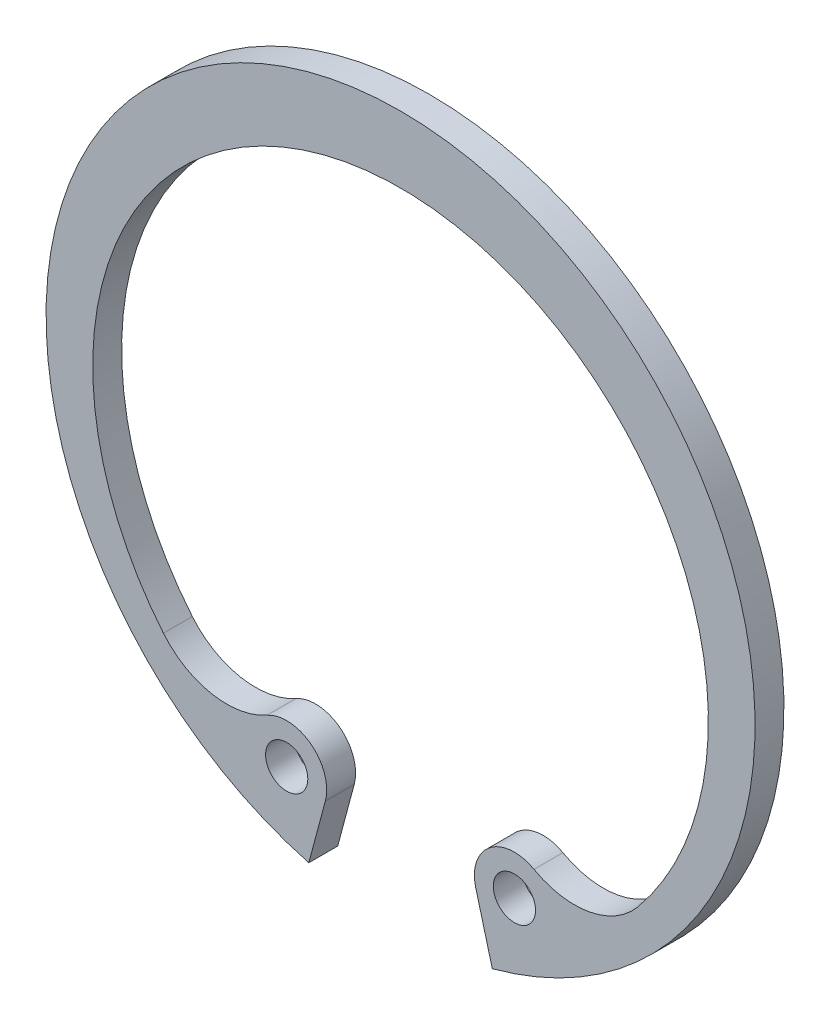
from build123d import *

# Parameters (mm, degrees)
SKETCH1_R           = 0.95
BOSS_EXTRUDE1_DEPTH = 1.3


with BuildPart() as part:
    # Sketch1 → Boss-Extrude1 (new body)
    with BuildSketch(Plane.XY):
        with BuildLine():
            ThreePointArc((-6.005563392, -9.696368719), (-4.019375294, -9.84339787), (-3.384498187, -11.731119191))
            Line((-3.384498187, -11.731119191), (-4.128163769, -14.506516929))
            ThreePointArc((-4.128163769, -14.506516929), (0, 16.85), (4.128163769, -14.506516929))
            Line((4.128163769, -14.506516929), (3.384498187, -11.731119191))
            ThreePointArc((3.384498187, -11.731119191), (4.019375294, -9.84339787), (6.005563392, -9.696368719))
            ThreePointArc((6.005563392, -9.696368719), (8.494705662, -10.109304713), (10.669798447, -8.830509674))
            ThreePointArc((10.669798447, -8.830509674), (0, 13.85), (-10.669798447, -8.830509674))
            ThreePointArc((-10.669798447, -8.830509674), (-8.494705662, -10.109304713), (-6.005563392, -9.696368719))
        make_face()
        with Locations((5.123164674, -11.26524491)):
            Circle(SKETCH1_R, mode=Mode.SUBTRACT)
        with Locations((-5.123164674, -11.26524491)):
            Circle(SKETCH1_R, mode=Mode.SUBTRACT)
    extrude(amount=BOSS_EXTRUDE1_DEPTH)


solid = part.part
